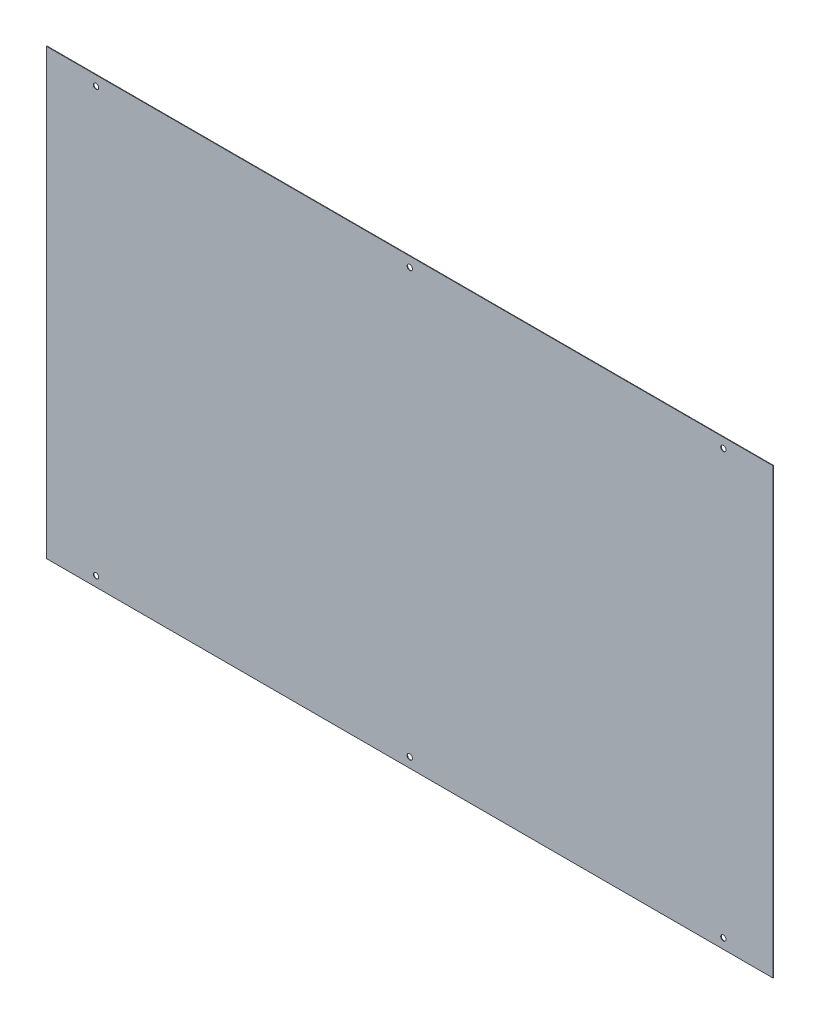
from build123d import *

# Parameters (mm, degrees)
SKETCH_1_W          = 1100
SKETCH_1_H          = 672
EXTRUDE_1_DEPTH     = 0.8
SKETCH_2_R          = 4
CUT_EXTRUDE_1_DEPTH = 0.8


with BuildPart() as part:
    # 草图1 → 凸台-拉伸1 (new body)
    with BuildSketch(Plane.XY):
        Rectangle(SKETCH_1_W, SKETCH_1_H)
    extrude(amount=EXTRUDE_1_DEPTH)

    # 草图2 → 切除-拉伸1 (cut)
    with BuildSketch(Plane(origin=(0, 0, 0), x_dir=(-1, 0, 0), z_dir=(0, 0, -1))):
        with Locations((0, 321)):
            Circle(SKETCH_2_R)
        with Locations((475, 321)):
            Circle(SKETCH_2_R)
        with Locations(Location((-475, 321, 0), (0, 0, 180))):
            Circle(SKETCH_2_R)
        with Locations((-475, -321)):
            Circle(SKETCH_2_R)
        with Locations(Location((475, -321, 0), (0, 0, 180))):
            Circle(SKETCH_2_R)
        with Locations(Location((0, -321, 0), (0, 0, 180))):
            Circle(SKETCH_2_R)
    extrude(amount=-CUT_EXTRUDE_1_DEPTH, mode=Mode.SUBTRACT)


solid = part.part
